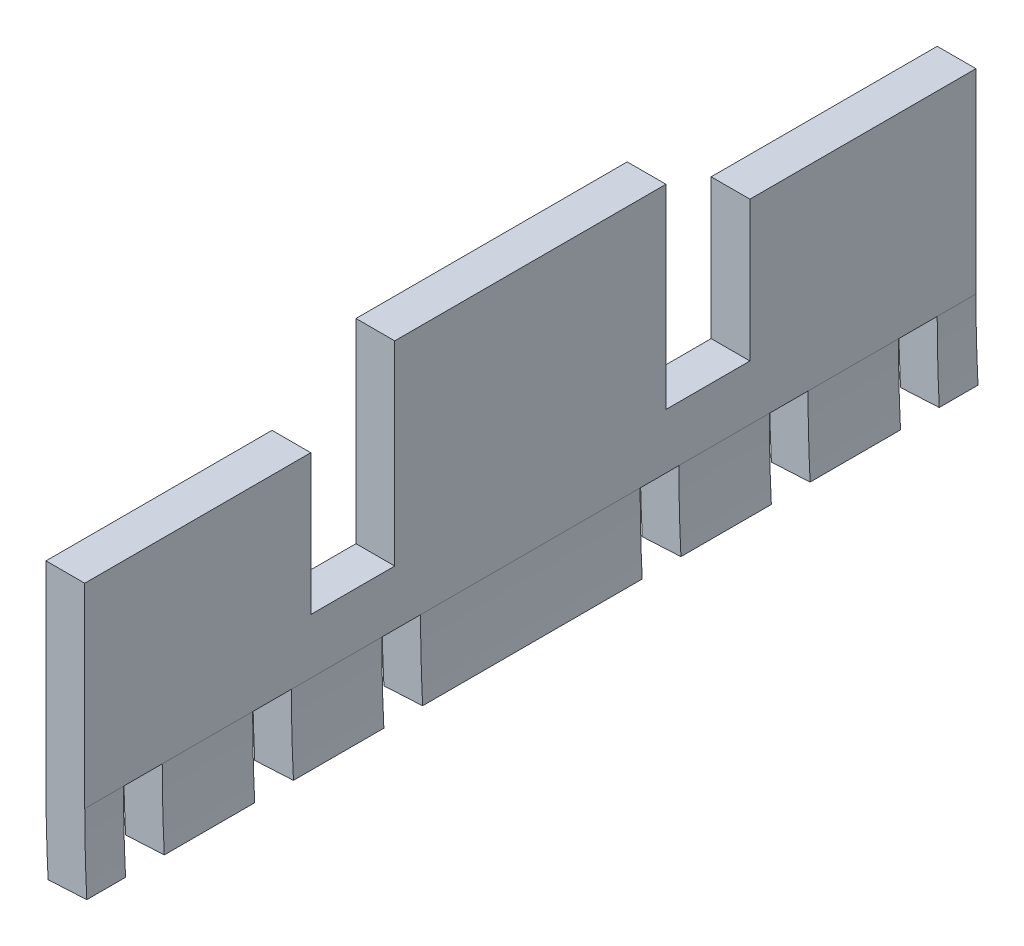
SolidWorks part; units mm, degrees
ref_plane "Front Plane" through (0, 0, 0) normal (0, 0, 1) x (1, 0, 0)
ref_plane "Top Plane" through (0, 0, 0) normal (0, 1, 0) x (1, 0, 0)
ref_plane "Right Plane" through (0, 0, 0) normal (1, 0, 0) x (0, 0, -1)
sketch "Sketch1" plane through (0, 0, 0) normal (0, 0, 1) x (1, 0, 0)
  line L0 (0, 0) -> (-437.5819, 0) construction
  line L1 (0, 0) -> (-350.4093, -18.3642) construction
  line L2 (-236.1759, -12.3775) -> (-230.1841, -12.0634)
  line L3 (-230.5, 0) -> (-230.5, 38.7225)
  line L4 (-236.5, 0) -> (-236.5, 38.7225)
  line L5 (-236.5, 38.7225) -> (-230.5, 38.7225)
  arc A0 (-236.5, 0) -> (-236.1759, -12.3775) centre (0, 0) ccw
  arc A1 (-230.5, 0) -> (-230.1841, -12.0634) centre (0, 0) ccw
  dimension "D1" = 461
  dimension "D2" = 473
  dimension "D3" = 3
  dimension "D4" = 51.1
extrude "Boss-Extrude1" add sketch "Sketch1" along normal mid plane 138
sketch "Sketch5" plane through (0, 0, 0) normal (1, 0, 0) x (0, 0, -1)
  line L0 (0, 0) -> (0, -54.0648) construction
  line L1 (-69, 0) -> (69, 0) construction
  line L2 (-63, -28.7498) -> (-57, -28.7498)
  line L3 (-63, -28.7498) -> (-63, 0)
  line L4 (-63, 0) -> (-57, 0)
  line L5 (-57, -28.7498) -> (-57, 0)
  line L6 (-69, 0) -> (-69, -12.0634) construction
  line L7 (-43, -28.7498) -> (-37, -28.7498)
  line L8 (-43, -28.7498) -> (-43, 0)
  line L9 (-43, 0) -> (-37, 0)
  line L10 (-37, -28.7498) -> (-37, 0)
  line L11 (-23, -28.7498) -> (-17, -28.7498)
  line L12 (-23, -28.7498) -> (-23, 0)
  line L13 (-23, 0) -> (-17, 0)
  line L14 (-17, -28.7498) -> (-17, 0)
  line L15 (17, -28.7498) -> (17, 0)
  line L16 (23, 0) -> (17, 0)
  line L17 (23, -28.7498) -> (23, 0)
  line L18 (23, -28.7498) -> (17, -28.7498)
  line L19 (37, -28.7498) -> (37, 0)
  line L20 (43, 0) -> (37, 0)
  line L21 (43, -28.7498) -> (43, 0)
  line L22 (43, -28.7498) -> (37, -28.7498)
  line L23 (57, -28.7498) -> (57, 0)
  line L24 (63, 0) -> (57, 0)
  line L25 (63, -28.7498) -> (63, 0)
  line L26 (63, -28.7498) -> (57, -28.7498)
  dimension "D1" = 6
  dimension "D2" = 6
  dimension "D3" = 14
  dimension "D4" = 40
extrude "Cut-Extrude5" cut sketch "Sketch5" against normal through all
sketch "Sketch3" plane through (-230.5, 0, 0) normal (1, 0, 0) x (0, 0, -1)
  line L0 (0, 38.7225) -> (0, 14.6129) construction
  line L1 (-69, 38.7225) -> (69, 38.7225) construction
  line L2 (-69, 30.2225) -> (-34, 30.2225)
  line L3 (-69, 0) -> (-69, 38.7225) construction
  line L4 (-34, 30.2225) -> (-34, 8.5225)
  line L5 (-34, 8.5225) -> (-21, 8.5225)
  line L6 (-21, 8.5225) -> (-21, 38.7225)
  line L7 (-69, 30.2225) -> (-69, 38.7225)
  line L8 (-69, 38.7225) -> (-21, 38.7225)
  line L9 (21, 8.5225) -> (21, 38.7225)
  line L10 (69, 38.7225) -> (21, 38.7225)
  line L11 (69, 30.2225) -> (69, 38.7225)
  line L12 (34, 8.5225) -> (21, 8.5225)
  line L13 (34, 30.2225) -> (34, 8.5225)
  line L14 (69, 30.2225) -> (34, 30.2225)
  dimension "D1" = 35
  dimension "D2" = 13
  dimension "D3" = 30.2
  dimension "D4" = 8.5
extrude "Cut-Extrude1" cut sketch "Sketch3" against normal through all
